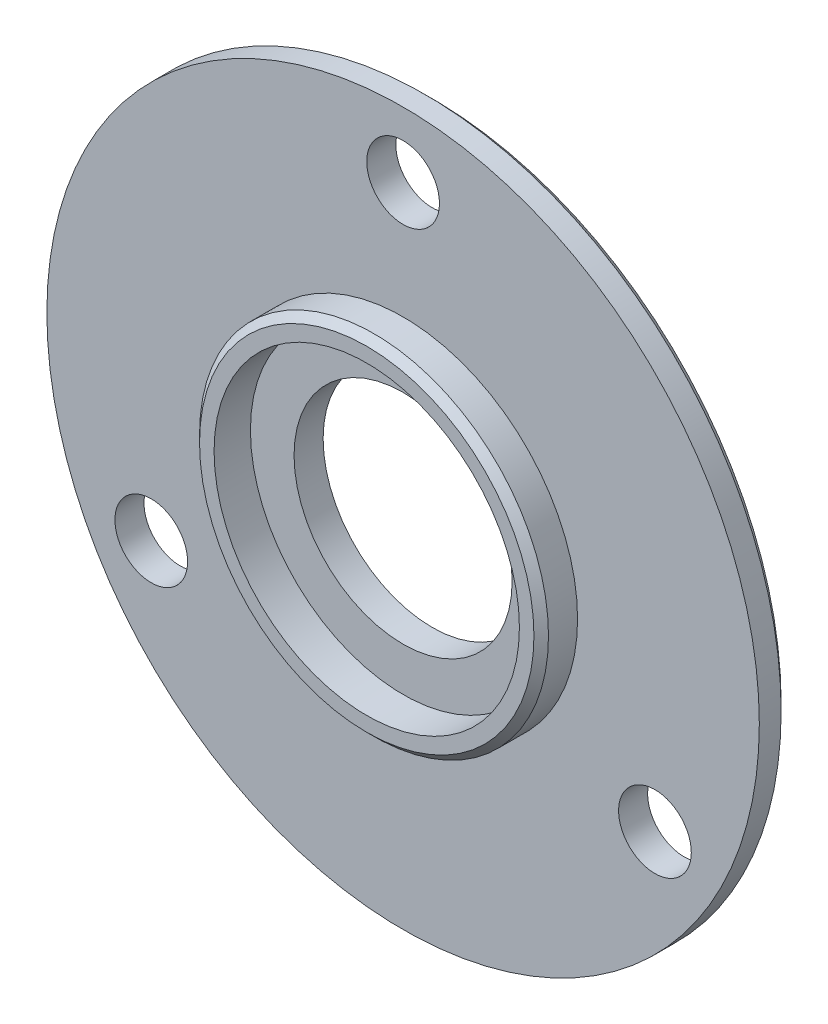
from build123d import *

# Parameters (mm, degrees)
SKETCH1_R           = 24.5
BOSS_EXTRUDE1_DEPTH = 2
SKETCH2_R           = 12
BOSS_EXTRUDE2_DEPTH = 2.5
CUT_EXTRUDE1_START  = 2.5
SKETCH3_R           = 10.5
CUT_EXTRUDE1_DEPTH  = 2.5
SKETCH4_R           = 7.5
CUT_EXTRUDE2_DEPTH  = 2.5
SKETCH5_R           = 2.5
CUT_EXTRUDE3_DEPTH  = 2.5
CHAMFER1_SIZE       = 0.5


with BuildPart() as part:
    # Sketch1 → Boss-Extrude1 (new body)
    with BuildSketch(Plane.XY):
        Circle(SKETCH1_R)
    extrude(amount=BOSS_EXTRUDE1_DEPTH)

    # Sketch2 → Boss-Extrude2 (add)
    with BuildSketch(Plane.XY.offset(2)):
        Circle(SKETCH2_R)
    extrude(amount=BOSS_EXTRUDE2_DEPTH)

    # Sketch3 → Cut-Extrude1 (cut)
    with BuildSketch(Plane.XY.offset(2).offset(CUT_EXTRUDE1_START)):
        Circle(SKETCH3_R)
    extrude(amount=-CUT_EXTRUDE1_DEPTH, mode=Mode.SUBTRACT)

    # Sketch4 → Cut-Extrude2 (cut)
    with BuildSketch(Plane.XY.offset(2)):
        Circle(SKETCH4_R)
    extrude(amount=-CUT_EXTRUDE2_DEPTH, mode=Mode.SUBTRACT)

    # Sketch5 → Cut-Extrude3 (cut)
    with BuildSketch(Plane.XY.offset(2)):
        with Locations((0, 20)):
            Circle(SKETCH5_R)
        with Locations((17.320508076, -10)):
            Circle(SKETCH5_R)
        with Locations((-17.320508076, -10)):
            Circle(SKETCH5_R)
    extrude(amount=-CUT_EXTRUDE3_DEPTH, mode=Mode.SUBTRACT)

    # Chamfer1
    chamfer1_edges = [part.edges().sort_by_distance(p)[0] for p in [
        (-24.5, 0, 0),
        (-12, 0, 4.5),
    ]]
    chamfer(chamfer1_edges, length=CHAMFER1_SIZE)


solid = part.part
